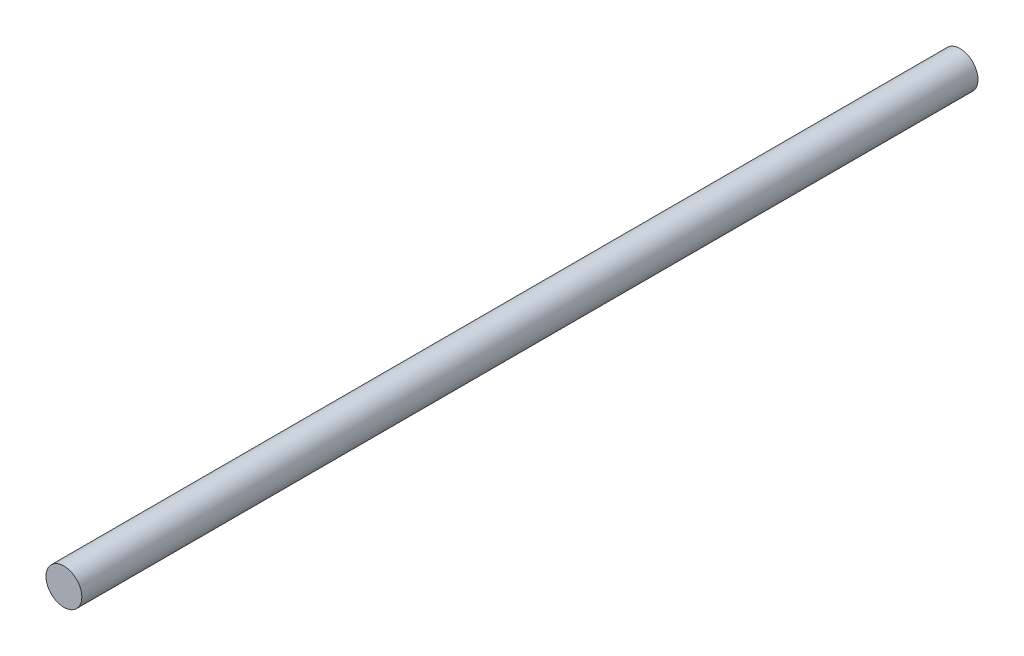
from build123d import *

# Parameters (mm, degrees)
SKETCH1_R           = 5
BOSS_EXTRUDE1_DEPTH = 250


with BuildPart() as part:
    # Sketch1 → Boss-Extrude1 (new body)
    with BuildSketch(Plane.XY):
        Circle(SKETCH1_R)
    extrude(amount=BOSS_EXTRUDE1_DEPTH)


solid = part.part
